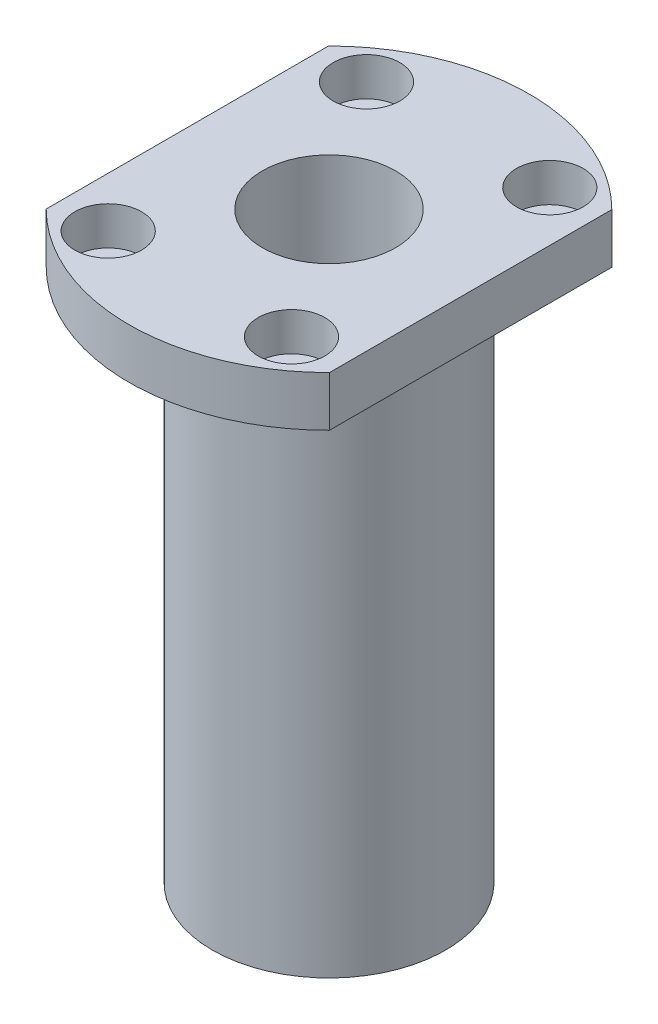
from build123d import *

# Parameters (mm, degrees)
SKETCH1_R                                            = 14
BOSS_EXTRUDE1_DEPTH                                  = 64
SKETCH2_R                                            = 24
BOSS_EXTRUDE2_DEPTH                                  = 6
SKETCH3_OUTSIDE_W                                    = 69.502
SKETCH3_OUTSIDE_H                                    = 69.502
CUT_EXTRUDE2_DEPTH                                   = 6
SKETCH4_R                                            = 8
CUT_EXTRUDE3_DEPTH                                   = 76.927597091
HOLE_SIZE_PER_SOCKET_HEAD_CAP_SCREW_TYPE_D           = 4.5
HOLE_SIZE_PER_SOCKET_HEAD_CAP_SCREW_TYPE_CBORE_D     = 8
HOLE_SIZE_PER_SOCKET_HEAD_CAP_SCREW_TYPE_CBORE_DEPTH = 4.6


with BuildPart() as part:
    # Sketch1 → Boss-Extrude1 (new body)
    with BuildSketch(Plane(origin=(0, 0, 0), x_dir=(1, 0, 0), z_dir=(0, 1, 0))):
        with Locations(Location((0, 0, 0), (0, 0, 270))):
            Circle(SKETCH1_R)
    extrude(amount=BOSS_EXTRUDE1_DEPTH)

    # Sketch2 → Boss-Extrude2 (add)
    with BuildSketch(Plane(origin=(0, 64, 0), x_dir=(1, 0, 0), z_dir=(0, 1, 0))):
        with Locations(Location((0, 0, 0), (0, 0, 270))):
            Circle(SKETCH2_R)
    extrude(amount=BOSS_EXTRUDE2_DEPTH)

    # Sketch3 outside → Cut-Extrude2 (cut)
    with BuildSketch(Plane(origin=(0, 70, 0), x_dir=(1, 0, 0), z_dir=(0, 1, 0))):
        Rectangle(SKETCH3_OUTSIDE_W, SKETCH3_OUTSIDE_H)
        with BuildLine():
            Line((-17, 16.941074346), (-17, -16.941074346))
            ThreePointArc((-17, -16.941074346), (0, -24), (17, -16.941074346))
            Line((17, -16.941074346), (17, 16.941074346))
            ThreePointArc((17, 16.941074346), (0, 24), (-17, 16.941074346))
        make_face(mode=Mode.SUBTRACT)
    extrude(amount=-CUT_EXTRUDE2_DEPTH, mode=Mode.SUBTRACT)

    # Sketch4 → Cut-Extrude3 (cut, through all)
    with BuildSketch(Plane.XZ):
        with Locations(Location((0, 0, 0), (0, 0, 270))):
            Circle(SKETCH4_R)
    extrude(amount=-CUT_EXTRUDE3_DEPTH, mode=Mode.SUBTRACT)

    # Hole size per socket head cap screw type1 (through all)
    with Locations(Plane(origin=(0, 70, 0), x_dir=(-1, 0, 0), z_dir=(0, 1, 0))):
        with Locations((-11, 15.5), (11, 15.5), (11, -15.5), (-11, -15.5)):
            CounterBoreHole(HOLE_SIZE_PER_SOCKET_HEAD_CAP_SCREW_TYPE_D / 2, HOLE_SIZE_PER_SOCKET_HEAD_CAP_SCREW_TYPE_CBORE_D / 2, HOLE_SIZE_PER_SOCKET_HEAD_CAP_SCREW_TYPE_CBORE_DEPTH)


solid = part.part
